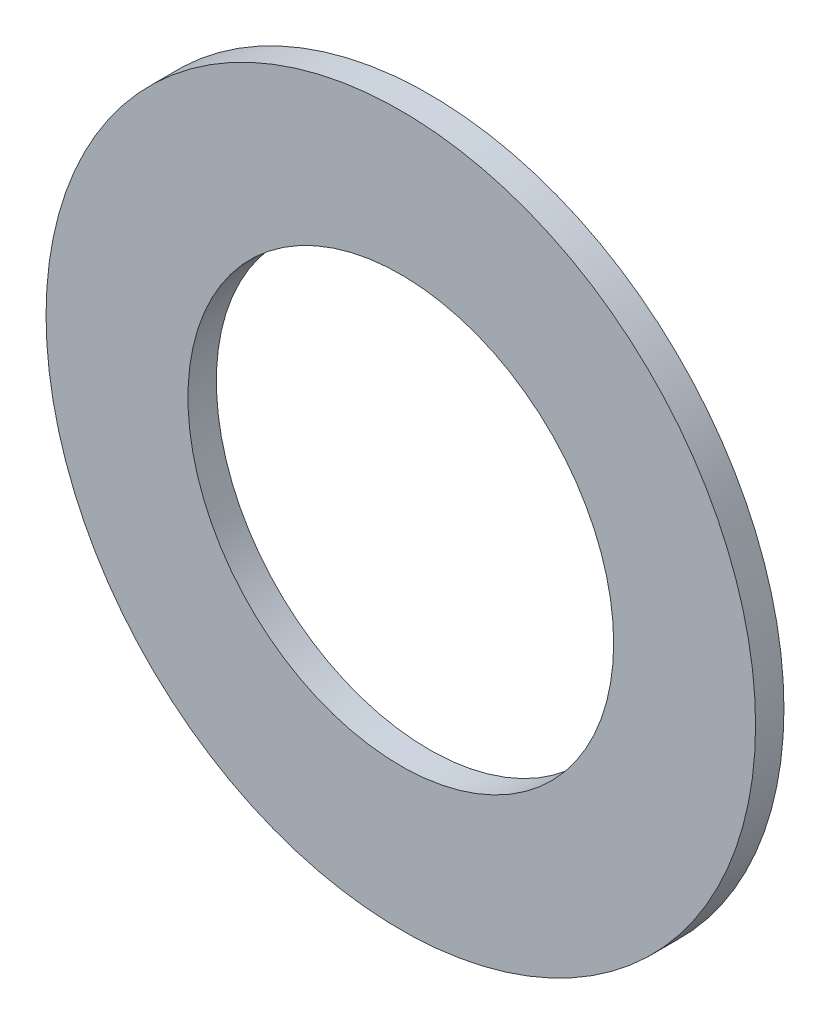
from build123d import *

# Parameters (mm, degrees)
SKETCH_1_R      = 15
SKETCH_1_R_2    = 9
EXTRUDE_1_DEPTH = 1.2


with BuildPart() as part:
    # 草图1 → 凸台-拉伸1 (new body)
    with BuildSketch(Plane.XY):
        with Locations((-3.15038311, -4.2341149)):
            Circle(SKETCH_1_R)
        with Locations((-3.15038311, -4.2341149)):
            Circle(SKETCH_1_R_2, mode=Mode.SUBTRACT)
    extrude(amount=EXTRUDE_1_DEPTH)


solid = part.part
